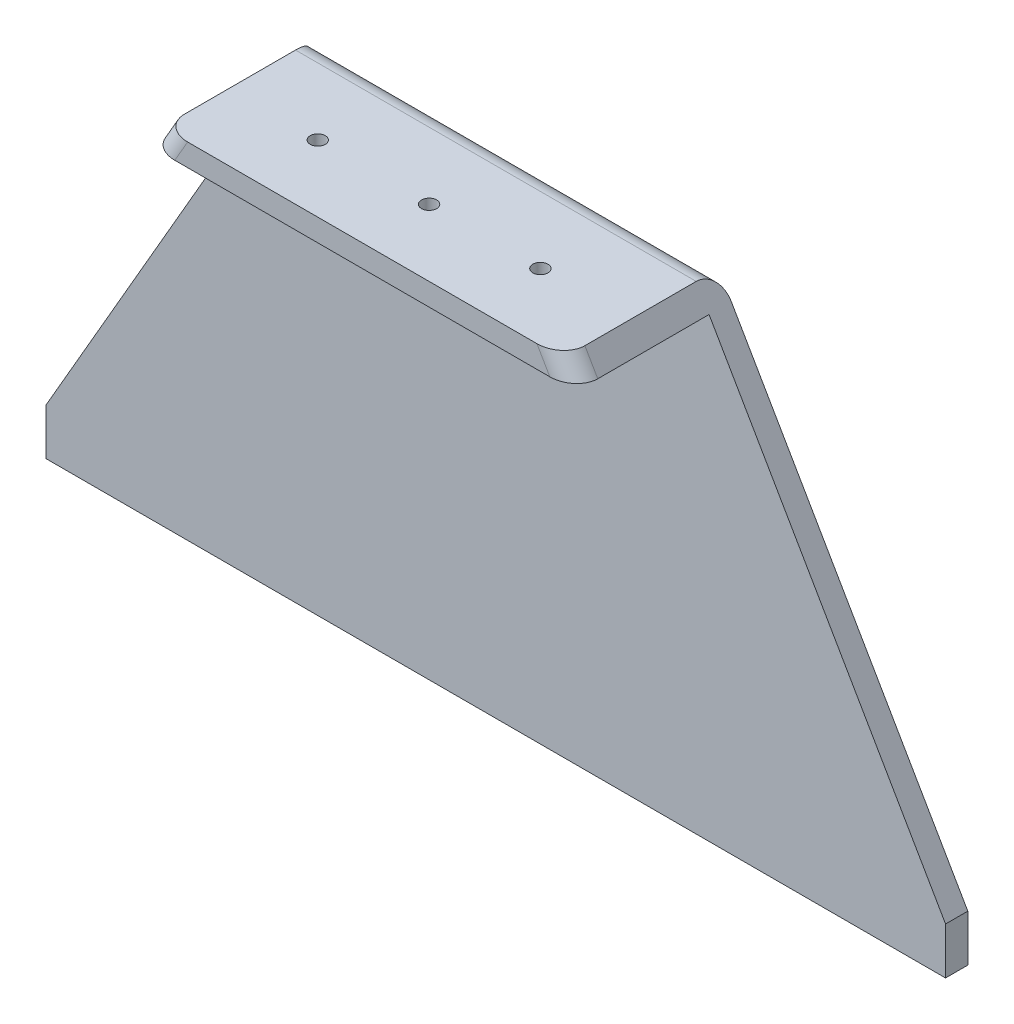
SolidWorks part; units mm, degrees
material "1023 碳钢板 (SS)"
ref_plane "前视基准面" through (0, 0, 0) normal (0, 0, 1) x (1, 0, 0)
ref_plane "上视基准面" through (0, 0, 0) normal (0, 1, 0) x (1, 0, 0)
ref_plane "右视基准面" through (0, 0, 0) normal (1, 0, 0) x (0, 0, -1)
sketch "草图1" plane through (0, 0, 0) normal (0, 0, 1) x (1, 0, 0)
  line L1 (-202, 107.5) -> (202, 107.5)
  line L2 (-202, 107.5) -> (-202, -107.5)
  line L3 (-202, -107.5) -> (202, -107.5)
  line L4 (202, 107.5) -> (202, -107.5)
  line L5 (-202, 107.5) -> (202, -107.5) construction
  line L6 (-202, -107.5) -> (202, 107.5) construction
  point P0 (0, 0)
  dimension "D1" = 404
  dimension "D2" = 215
extrude "凸台-拉伸1" add sketch "草图1" along normal blind 70
shell "抽壳1" thickness 10
sketch "草图2" plane through (0, 0, 70) normal (0, 0, 1) x (1, 0, 0)
  line L0 (-202, -86.4897) -> (-90, 107.5)
  line L1 (-202, 107.5) -> (-202, -107.5) construction
  line L2 (202, 107.5) -> (-202, 107.5) construction
  line L3 (-90, 107.5) -> (-202, 107.5)
  line L4 (-202, 107.5) -> (-202, -86.4897)
  line L5 (0, 0) -> (0, 147.2123) construction
  line L6 (90, 107.5) -> (202, 107.5)
  line L7 (202, -86.4897) -> (90, 107.5)
  line L8 (202, 107.5) -> (202, -86.4897)
  dimension "D1" = 180
  dimension "D2" = 60
extrude "切除-拉伸1" cut sketch "草图2" against normal blind 80
sketch "草图6" plane through (0, -107.5, 0) normal (0, -1, 0) x (1, 0, 0)
  line L0 (-202, 70) -> (-202, 0) construction
  line L1 (-642.9627, 10) -> (238.9627, 10)
  line L2 (-642.9627, 10) -> (-642.9627, 177.7152)
  line L3 (-642.9627, 177.7152) -> (238.9627, 177.7152)
  line L4 (238.9627, 10) -> (238.9627, 177.7152)
  line L5 (-642.9627, 10) -> (238.9627, 177.7152) construction
  line L6 (-642.9627, 177.7152) -> (238.9627, 10) construction
  line L7 (-202, 0) -> (202, 0) construction
  point P0 (-202, 93.8576)
  point P7 (-202, 102.622)
  dimension "D1" = 10
extrude "切除-拉伸2" cut sketch "草图6" against normal blind 205
sketch "草图3" plane through (0, 107.5, 0) normal (0, 1, 0) x (1, 0, 0)
  line L0 (-90, 0) -> (-90, -70) construction
  line L5 (90, 0) -> (-90, 0) construction
  circle A0 centre (-50, -40) radius 13.2407
  circle A1 centre (0, -40) radius 14.1864
  circle A2 centre (50, -40) radius 12.6102
  point P10 (0, 0)
  dimension "D4" = 40
  dimension "D1" = 50
  dimension "D2" = 50
  dimension "D3" = 40
hole_wizard "M8 螺纹孔1" positions "草图4" profile "草图5" tap size "M8" standard "ISO"
sketch "草图4" plane through (0, 107.5, 0) normal (0, 1, 0) x (1, 0, 0)
  point P0 (-50, -40)
  point P3 (0, -40)
  point P6 (50, -40)
sketch "草图5" plane through (-50, 107.5, 40) normal (1, 0, 0) x (0, 0, 1)
  line L0 (0, 0) -> (0, 21.7929)
  line L1 (0, 21.7929) -> (3.4, 19.75)
  line L2 (3.4, 19.75) -> (3.4, 0)
  line L5 (3.4, 0) -> (0, 0)
  line L10 (0, 21.7929) -> (-3.4, 19.75) construction
  line L11 (0, -6.35) -> (0, 107.95) construction
  dimension "螺纹孔钻头直径" = 6.8
  dimension "螺纹孔钻头深度" = 19.75
  dimension "导头角度" = 118
cosmetic thread "孔螺蚊线1" parameters "D1"=16, "D2"=8
cosmetic thread "孔螺蚊线2" parameters "D1"=16, "D2"=8
cosmetic thread "孔螺蚊线3" parameters "D1"=16, "D2"=8
fillet "圆角1" radius 10 3 edges at (0, 107.5, 0) (92.8868, 102.5, 70) (-92.8868, 102.5, 70)
